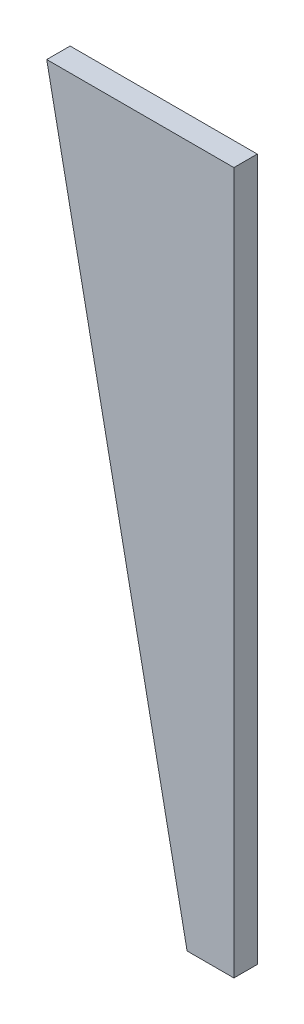
from build123d import *

# Parameters (mm, degrees)
EXTRUDE1_DEPTH = 5


with BuildPart() as part:
    # Sketch1 → Extrude1 (new, symmetric)
    with BuildSketch(Plane.XY):
        Polygon((-80, 0), (0, 0), (0, -300), (-20, -300), align=None)
    extrude(amount=EXTRUDE1_DEPTH, both=True)


solid = part.part
